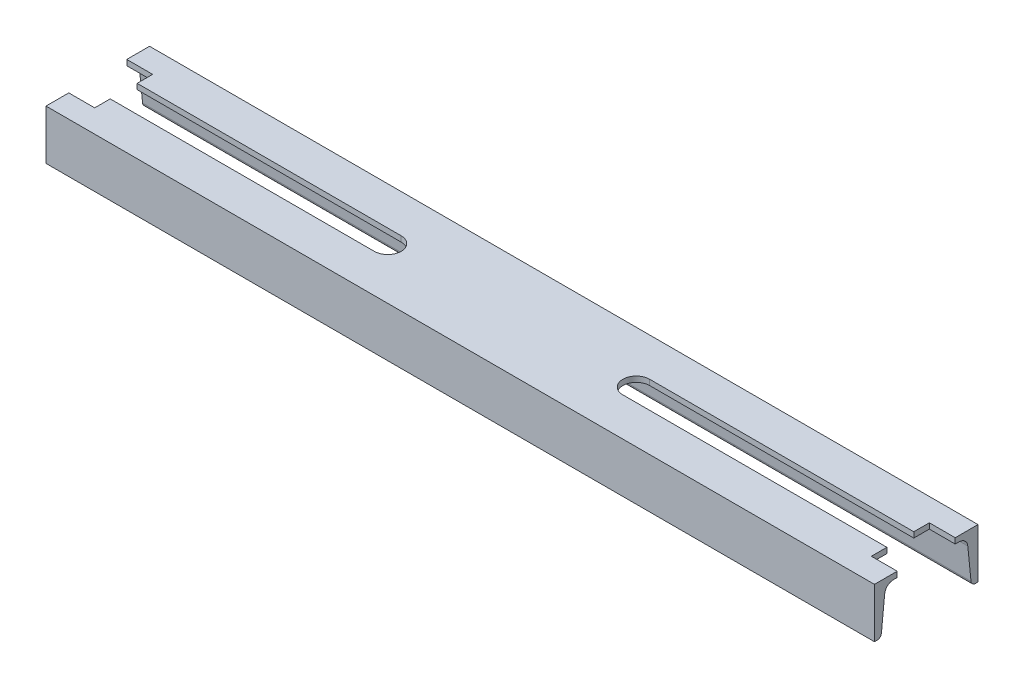
from build123d import *

# Parameters (mm, degrees)
HOT_ROLLED_CHANNEL_STEEL_GB_T_707_1988_DEPTH = 800
CUT_EXTRUDE1_DEPTH                           = 10
SKETCH4_W                                    = 25
SKETCH4_H                                    = 15
CUT_EXTRUDE2_DEPTH                           = 10


with BuildPart() as part:
    # Sketch1 → hot-rolled channel steel (GB/T 707-1988) 10(1) (new body)
    with BuildSketch(Plane(origin=(400, 0, 0), x_dir=(0, -1, 0), z_dir=(-1, 0, 0))):
        with BuildLine():
            Line((48, 100), (0, 100))
            Line((0, 100), (0, 0))
            Line((0, 0), (48, 0))
            Line((48, 0), (48, 2.518802861))
            ThreePointArc((48, 2.518802861), (46.901173268, 5.370575474), (44.172890806, 6.747710919))
            Line((44.172890806, 6.747710919), (12.954218388, 9.869578161))
            ThreePointArc((12.954218388, 9.869578161), (7.497653465, 12.623849051), (5.3, 18.327394278))
            Line((5.3, 18.327394278), (5.3, 81.672605722))
            ThreePointArc((5.3, 81.672605722), (7.497653465, 87.376150949), (12.954218388, 90.130421839))
            Line((12.954218388, 90.130421839), (44.172890806, 93.252289081))
            ThreePointArc((44.172890806, 93.252289081), (46.901173268, 94.629424526), (48, 97.481197139))
            Line((48, 97.481197139), (48, 100))
        make_face()
    extrude(amount=HOT_ROLLED_CHANNEL_STEEL_GB_T_707_1988_DEPTH)

    # Sketch3 → Cut-Extrude1 (cut)
    with BuildSketch(Plane(origin=(0, 0, 0), x_dir=(1, 0, 0), z_dir=(0, 1, 0))):
        with BuildLine():
            Line((-680, -37), (-120, -37))
            ThreePointArc((-120, -37), (-107, -50), (-120, -63))
            Line((-120, -63), (-680, -63))
            ThreePointArc((-680, -63), (-693, -50), (-680, -37))
        make_face()
    cut_extrude1 = extrude(amount=-CUT_EXTRUDE1_DEPTH, mode=Mode.SUBTRACT)

    # Sketch4 → Cut-Extrude2 (cut)
    with BuildSketch(Plane(origin=(0, 0, 0), x_dir=(1, 0, 0), z_dir=(0, 1, 0))):
        with Locations((-387.5, -29.5)):
            Rectangle(SKETCH4_W, SKETCH4_H)
        with Locations((-387.5, -70.5)):
            Rectangle(SKETCH4_W, SKETCH4_H)
    cut_extrude2 = extrude(amount=-CUT_EXTRUDE2_DEPTH, mode=Mode.SUBTRACT)

    # Mirror1: Cut-Extrude1, Cut-Extrude2 across plane
    add(cut_extrude1.mirror(Plane(origin=(0, 0, 0), x_dir=(0, 0, 1), z_dir=(1, 0, 0))), mode=Mode.SUBTRACT)
    add(cut_extrude2.mirror(Plane(origin=(0, 0, 0), x_dir=(0, 0, 1), z_dir=(1, 0, 0))), mode=Mode.SUBTRACT)


solid = part.part
